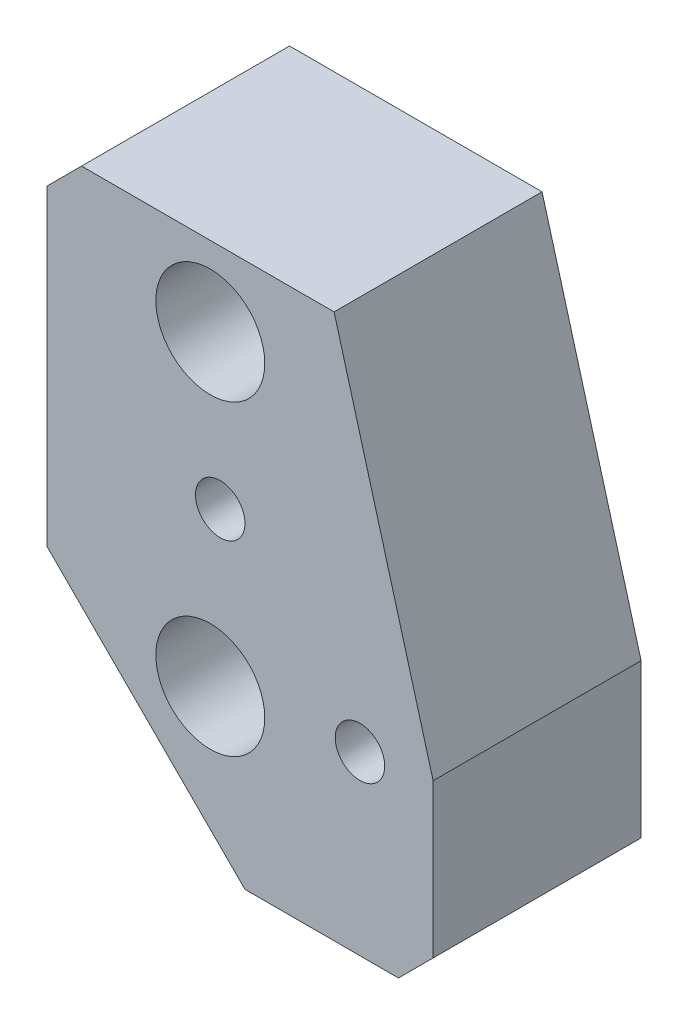
from build123d import *

# Parameters (mm, degrees)
EXTRUDE_1_DEPTH        = 21
SKETCH_2_R             = 5.5
CUT_EXTRUDE_1_DEPTH    = 9
SKETCH_3_R             = 3.5
CUT_EXTRUDE_2_DEPTH    = 69.483574673
HOLE_WIZARD_M6_1_D     = 5
HOLE_WIZARD_M6_1_DEPTH = 17
HOLE_WIZARD_M6_1_TIP   = 1.502151548


with BuildPart() as part:
    # 草图1 → 凸台-拉伸1 (new body)
    with BuildSketch(Plane.XY):
        Polygon((0, 20), (20, 0), (35.5, 0), (39, 3.5), (39, 19), (29, 55), (3.5, 55), (0, 51.5), align=None)
    extrude(amount=EXTRUDE_1_DEPTH)

    # 草图2 → 切除-拉伸1 (cut)
    with BuildSketch(Plane.XY.offset(21)):
        with Locations((16.5, 47)):
            Circle(SKETCH_2_R)
        with Locations((16.5, 16)):
            Circle(SKETCH_2_R)
    extrude(amount=-CUT_EXTRUDE_1_DEPTH, mode=Mode.SUBTRACT)

    # 草图3 → 切除-拉伸2 (cut, through all)
    with BuildSketch(Plane.XY.offset(12)):
        with Locations((16.5, 47)):
            Circle(SKETCH_3_R)
        with Locations((16.5, 16)):
            Circle(SKETCH_3_R)
    extrude(amount=-CUT_EXTRUDE_2_DEPTH, mode=Mode.SUBTRACT)

    # M6 螺纹孔1
    with Locations(Plane(origin=(17.5, 32, 21), x_dir=(1, 0, 0), z_dir=(0, 0, 1))):
        with Locations((0, 0), (14.112362721, -14.171845978)):
            Hole(HOLE_WIZARD_M6_1_D / 2, depth=HOLE_WIZARD_M6_1_DEPTH)
            with Locations((0, 0, -(HOLE_WIZARD_M6_1_DEPTH + HOLE_WIZARD_M6_1_TIP / 2))):  # 118° drill point
                Cone(0, HOLE_WIZARD_M6_1_D / 2, HOLE_WIZARD_M6_1_TIP, mode=Mode.SUBTRACT)


solid = part.part
